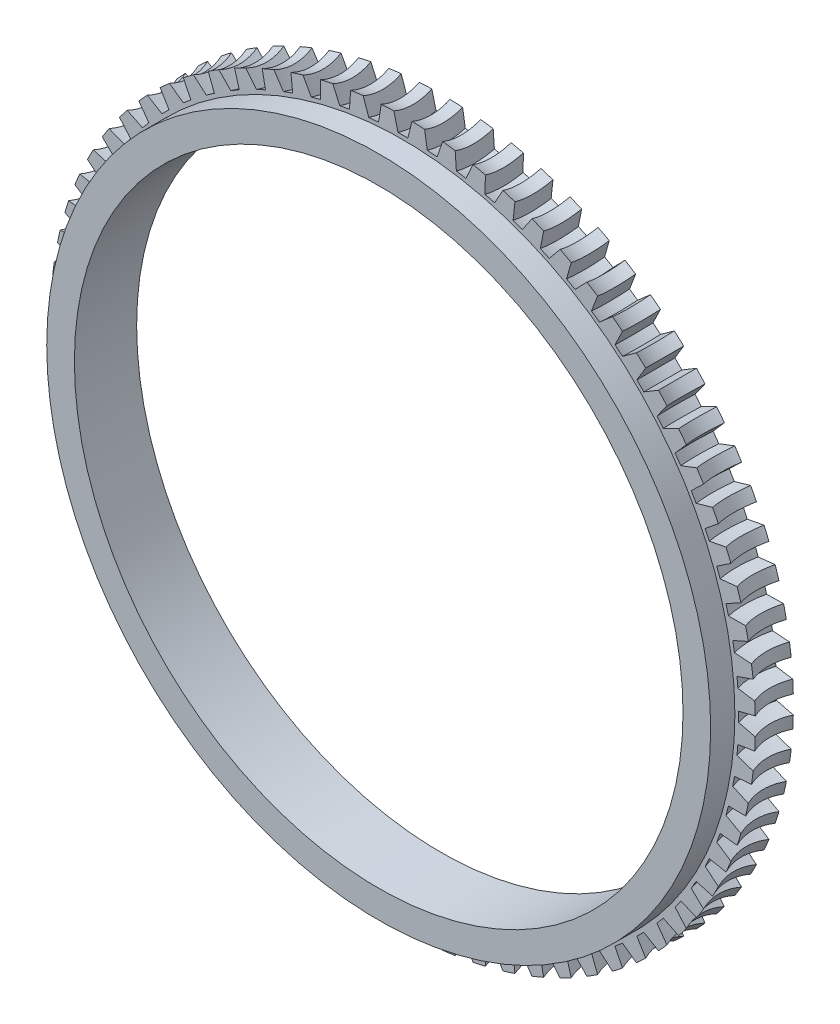
from build123d import *

# Parameters (mm, degrees)
CIRPATTERN1_COUNT = 72


with BuildPart() as part:
    # Sketch1 → Revolve1 (revolve)
    with BuildSketch(Plane(origin=(0, 318.5, 0), x_dir=(-1, 0, 0), z_dir=(0, -1, 0)), mode=Mode.PRIVATE) as revolve1_sk:
        with BuildLine():
            Line((176, 77.5), (192, 77.5))
            Line((192, 77.5), (192, 91.5))
            Line((192, 91.5), (203.842343988, 91.5))
            ThreePointArc((203.842343988, 91.5), (201.5, 102.5), (203.842343988, 113.5))
            Line((203.842343988, 113.5), (176, 113.5))
            Line((176, 113.5), (176, 77.5))
        make_face()
    revolve(revolve1_sk.sketch.rotate(Axis((0, 318.5, 0), (0, 0, -1)), 180), axis=Axis((0, 318.5, 0), (0, 0, -1)))

    # Cut-Sweep1: sweep along a path in Sketch3
    with BuildLine(Plane(origin=(0, 0, 0), x_dir=(0, 0, -1), z_dir=(1, 0, 0))) as cut_sweep1_path:
        ThreePointArc((121.95439119, 112.836958279), (102.250775003, 119.998964764), (82.668871119, 112.510582562))
    # Sketch2 → Cut-Sweep1 (sweep, cut)
    with BuildSketch(Plane(origin=(0, 0, -102.5), x_dir=(-1, 0, 0), z_dir=(0, 0, -1))):
        with BuildLine():
            Line((2.835709747, 126.020887496), (5.899857512, 114.585332354))
            ThreePointArc((5.899857512, 114.585332354), (0, 114.5), (-5.899857512, 114.585332354))
            Line((-5.899857512, 114.585332354), (-2.835709747, 126.020887496))
            ThreePointArc((-2.835709747, 126.020887496), (0, 126), (2.835709747, 126.020887496))
        make_face()
    cut_sweep1 = sweep(path=cut_sweep1_path.line, mode=Mode.SUBTRACT)

    # CirPattern1: Cut-Sweep1 ×72 about axis
    cirpattern1_axis = Axis((0, 318.5, 0), (0, 0, 1))
    for i in range(1, CIRPATTERN1_COUNT):
        add(cut_sweep1.rotate(cirpattern1_axis, i * 360 / CIRPATTERN1_COUNT), mode=Mode.SUBTRACT)


solid = part.part
